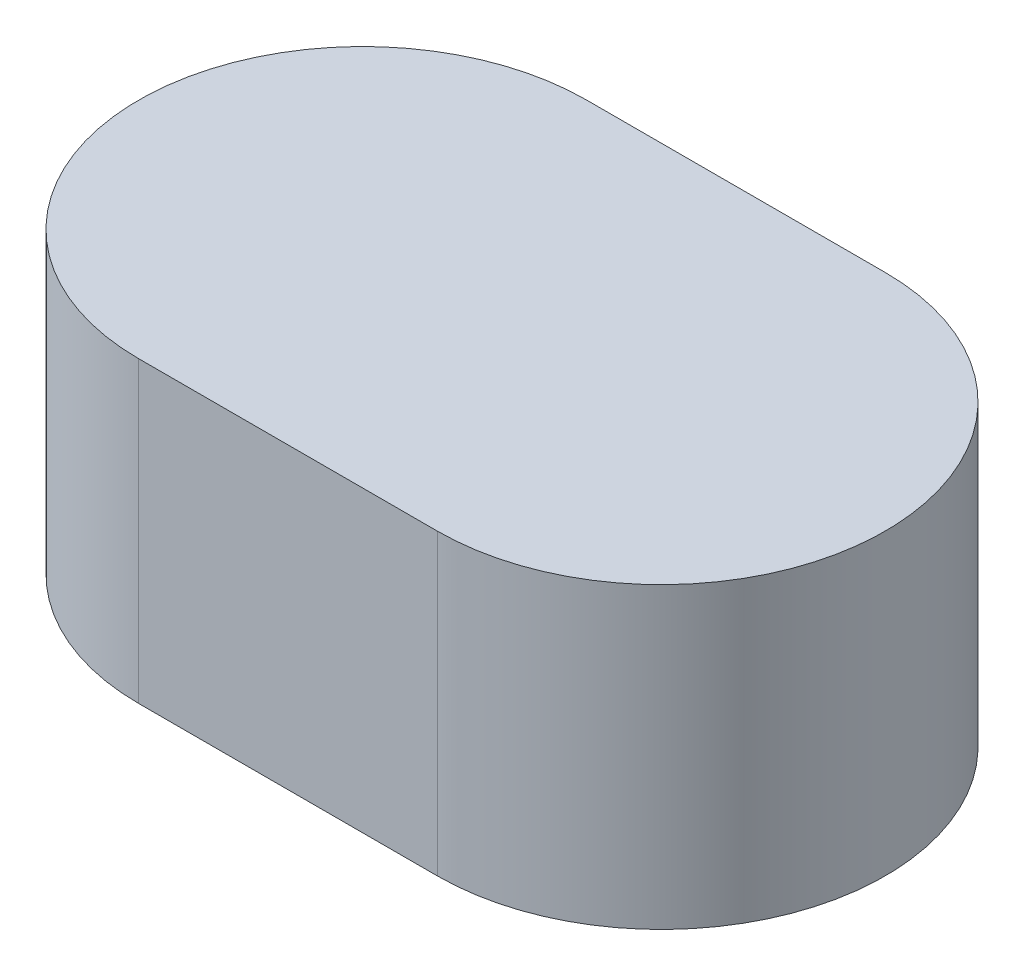
SolidWorks part; units mm, degrees
ref_plane "Front Plane" through (0, 0, 0) normal (0, 0, 1) x (1, 0, 0)
ref_plane "Top Plane" through (0, 0, 0) normal (0, 1, 0) x (1, 0, 0)
ref_plane "Right Plane" through (0, 0, 0) normal (1, 0, 0) x (0, 0, -1)
other "Configuration Table"
sketch "Sketch1" plane through (0, 0, 0) normal (0, 1, 0) x (1, 0, 0)
  line L0 (-4, 0) -> (4, 0) construction
  line L1 (-4, 6) -> (4, 6)
  line L2 (-4, -6) -> (4, -6)
  arc A0 (-4, 6) -> (-4, -6) centre (-4, 0) ccw
  arc A1 (4, -6) -> (4, 6) centre (4, 0) ccw
  point P2 (0, 0)
  dimension "D1" = 12
  dimension "D2" = 8
extrude "Boss-Extrude1" add sketch "Sketch1" along normal blind 8
